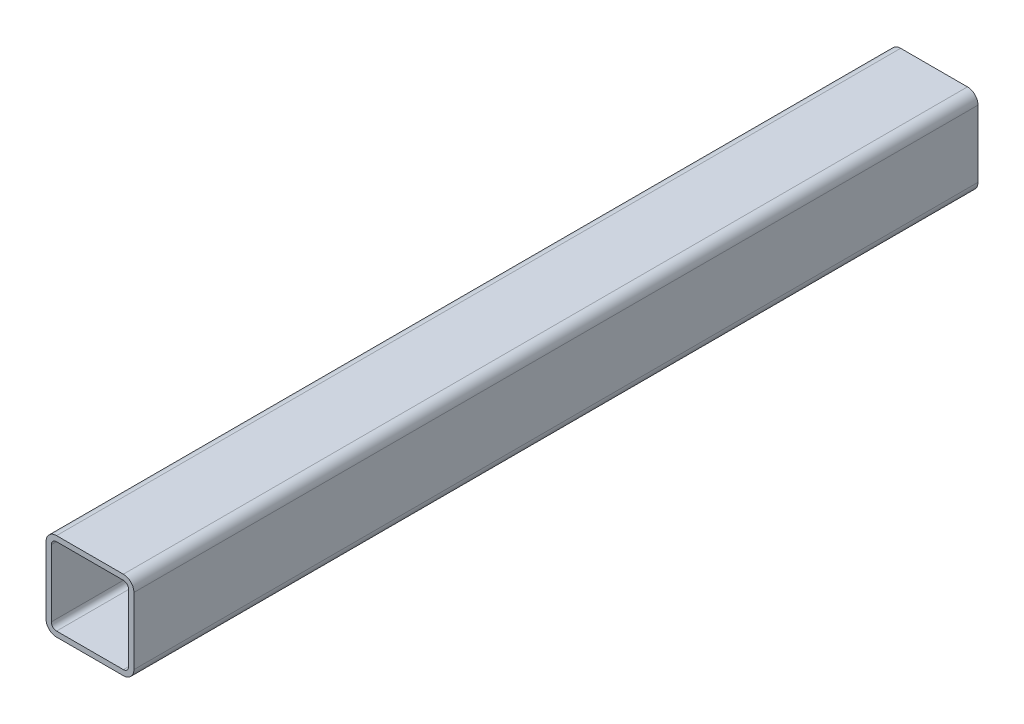
from build123d import *

# Parameters (mm, degrees)
GB_6728_1986_050_X_50_X_3_1_DEPTH = 480


with BuildPart() as part:
    # Sketch1 → Gb／6728-1986方形空心型钢 050 X 50 X 3(1) (new body)
    with BuildSketch(Plane(origin=(0, 0, 0), x_dir=(-1, 0, 0), z_dir=(0, 0, -1))):
        with BuildLine():
            Line((-19, -25), (19, -25))
            ThreePointArc((19, -25), (23.242640687, -23.242640687), (25, -19))
            Line((25, -19), (25, 19))
            ThreePointArc((25, 19), (23.242640687, 23.242640687), (19, 25))
            Line((19, 25), (-19, 25))
            ThreePointArc((-19, 25), (-23.242640687, 23.242640687), (-25, 19))
            Line((-25, 19), (-25, -19))
            ThreePointArc((-25, -19), (-23.242640687, -23.242640687), (-19, -25))
        make_face()
        with BuildLine():
            Line((-19, -22), (19, -22))
            ThreePointArc((19, -22), (21.121320344, -21.121320344), (22, -19))
            Line((22, -19), (22, 19))
            ThreePointArc((22, 19), (21.121320344, 21.121320344), (19, 22))
            Line((19, 22), (-19, 22))
            ThreePointArc((-19, 22), (-21.121320344, 21.121320344), (-22, 19))
            Line((-22, 19), (-22, -19))
            ThreePointArc((-22, -19), (-21.121320344, -21.121320344), (-19, -22))
        make_face(mode=Mode.SUBTRACT)
    extrude(amount=GB_6728_1986_050_X_50_X_3_1_DEPTH)


solid = part.part
